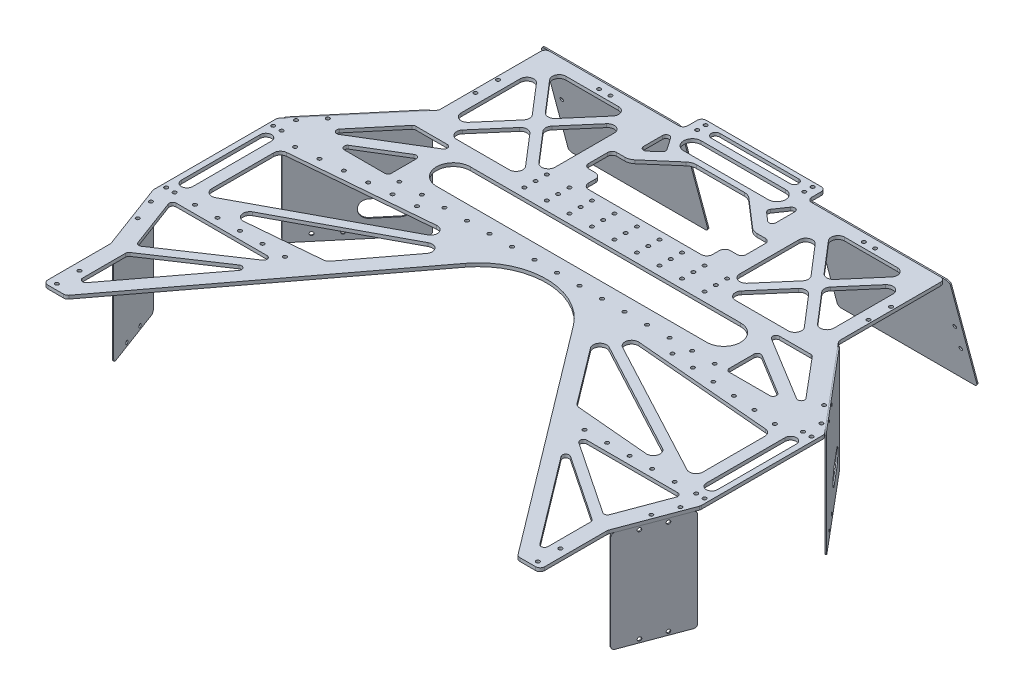
SolidWorks part; units mm, degrees
material "哈碳纤"
ref_plane "前视基准面" through (0, 0, 0) normal (0, 0, 1) x (1, 0, 0)
ref_plane "上视基准面" through (0, 0, 0) normal (0, 1, 0) x (1, 0, 0)
ref_plane "右视基准面" through (0, 0, 0) normal (1, 0, 0) x (0, 0, -1)
other "Configuration Table"
sketch "草图1" plane through (0, 0, 0) normal (0, 1, 0) x (1, 0, 0)
  line L0 (0, -705.937) -> (0, 34590.9145) construction
  line L1 (-55, 0) -> (55, 0)
  line L4 (177.5, -16.4193) -> (177.5, -111)
  line L5 (-177.5, -16.4193) -> (-177.5, -111)
  line L8 (177.5, -111) -> (243, -189)
  line L9 (-177.5, -111) -> (-243, -189)
  line L10 (243, -189) -> (243, -299)
  line L11 (-243, -189) -> (-243, -299)
  line L12 (243, -299) -> (220.55, -359)
  line L13 (-243, -299) -> (-220.55, -359)
  line L14 (220.55, -359) -> (220.55, -419)
  line L15 (-220.55, -359) -> (-220.55, -419)
  line L16 (220.55, -419) -> (200.55, -419)
  line L17 (-220.55, -419) -> (-200.55, -419)
  line L21 (239, -196.5) -> (239, -291.5) construction
  line L22 (-239, -196.5) -> (-239, -291.5) construction
  line L23 (200.55, -419) -> (47.8803, -216.841)
  line L24 (-200.55, -419) -> (-47.8803, -216.841)
  line L25 (234.9875, -309) -> (227.9787, -327.7317) construction
  line L26 (-234.9875, -309) -> (-227.9787, -327.7317) construction
  line L27 (220.3428, -166.684) -> (233.2043, -182) construction
  line L28 (-220.3428, -166.684) -> (-233.2043, -182) construction
  line L29 (217.8171, -159.0112) -> (213.2223, -162.8697) construction
  line L30 (213.2223, -162.8697) -> (234.1223, -187.7582) construction
  line L31 (234.1223, -187.7582) -> (238.7171, -183.8998) construction
  line L33 (55, 0) -> (55, -16.4193)
  line L34 (-55, 0) -> (-55, -16.4193)
  line L35 (55, -16.4193) -> (177.5, -16.4193)
  line L36 (-55, -16.4193) -> (-177.5, -16.4193)
  line L37 (177.5, -16.4193) -> (270.5, -16.4193) construction
  line L38 (270.5, -16.4193) -> (270.5, 8.5) construction
  line L39 (270.5, 8.5) -> (177.5, -16.4193) construction
  line L40 (270.5, -16.4193) -> (273.5, -16.4193) construction
  line L41 (273.5, -16.4193) -> (273.5, -15.6154) construction
  line L42 (273.5, -15.6154) -> (270.5, -16.4193) construction
  circle A0 centre (47.5, -4) radius 1.6
  circle A1 centre (-47.5, -4) radius 1.6
  circle A2 centre (47.5, -11.5) radius 1.6
  circle A3 centre (-47.5, -11.5) radius 1.6
  circle A4 centre (231.5, -196.5) radius 1.6
  circle A5 centre (-231.5, -196.5) radius 1.6
  circle A6 centre (239, -196.5) radius 1.6
  circle A7 centre (-239, -196.5) radius 1.6
  circle A8 centre (231.5, -291.5) radius 1.6
  circle A9 centre (-231.5, -291.5) radius 1.6
  circle A10 centre (239, -291.5) radius 1.6
  circle A11 centre (-239, -291.5) radius 1.6
  arc A12 (47.8803, -216.841) -> (-47.8803, -216.841) centre (0, -253) ccw
  circle A13 centre (213.55, -394) radius 1.6
  circle A14 centre (-213.55, -394) radius 1.6
  circle A15 centre (213.55, -414) radius 1.6
  circle A16 centre (-213.55, -414) radius 1.6
  circle A19 centre (234.9875, -309) radius 1.6
  circle A20 centre (227.9787, -327.7317) radius 1.6
  circle A21 centre (-227.9787, -327.7317) radius 1.6
  circle A22 centre (-234.9875, -309) radius 1.6
  circle A23 centre (220.3428, -166.684) radius 1.6
  circle A24 centre (233.2043, -182) radius 1.6
  circle A25 centre (-233.2043, -182) radius 1.6
  circle A26 centre (-220.3428, -166.684) radius 1.6
  circle A27 centre (112.5, -23.6154) radius 1.6
  circle A28 centre (122.5, -23.6154) radius 1.6
  circle A29 centre (-122.5, -23.6154) radius 1.6
  circle A30 centre (-112.5, -23.6154) radius 1.6
  circle A31 centre (174.5, -61.4193) radius 1.6
  circle A32 centre (174.5, -81.4193) radius 1.6
  circle A33 centre (-174.5, -81.4193) radius 1.6
  circle A34 centre (-174.5, -61.4193) radius 1.6
  point P6 (0, 0)
  point P24 (0, -318.0619)
  point P47 (239, -244)
  point P50 (243, -244)
extrude "凸台-拉伸1" add sketch "草图1" along normal blind 3
sketch "草图2" plane through (311.2944, 0, 116.476) normal (0.9366, 0, 0.3504) x (0.3504, 0, -0.9366)
  line L1 (-196.8824, 0) -> (-256.8824, 0)
  line L2 (-196.8824, 0) -> (-196.8824, -90)
  line L3 (-196.8824, -90) -> (-256.8824, -90)
  line L4 (-256.8824, 0) -> (-256.8824, -90)
  line L5 (-258.9449, 0) -> (-194.8824, 0) construction
  line L7 (-256.8824, -45) -> (-196.8824, -45) construction
  line L8 (-227.0561, 3) -> (-227.0561, 0) construction
  line L9 (-194.8824, 3) -> (-194.8824, 0) construction
  circle A0 centre (-237.0561, -3) radius 1.6
  circle A1 centre (-217.0561, -3) radius 1.6
  circle A2 centre (-217.0561, -87) radius 1.6
  circle A3 centre (-237.0561, -87) radius 1.6
  dimension "D3" = 3
  dimension "D4" = 3.2
  dimension "D1" = 90
  dimension "D2" = 60
  dimension "D5" = 20
  dimension "D6" = 10
  dimension "D7" = 2
extrude "凸台-拉伸2" add sketch "草图2" against normal blind 1 separate body
sketch "草图3" plane through (49.4311, 0, -41.5095) normal (0.7658, 0, -0.6431) x (-0.6431, 0, -0.7658)
  line L0 (-301.0042, 3) -> (-199.1501, 3) construction
  line L1 (-298.0042, 3) -> (-203.0042, 3)
  line L2 (-298.0042, 3) -> (-298.0042, -93)
  line L3 (-298.0042, -93) -> (-203.0042, -93)
  line L4 (-203.0042, 3) -> (-203.0042, -93)
  line L5 (-301.0042, 3) -> (-301.0042, 0) construction
  line L6 (-298.0042, -45) -> (-203.0042, -45) construction
  line L7 (-289.3442, 3) -> (-289.3442, 0) construction
  circle A0 centre (-279.3442, -3) radius 1.6
  circle A1 centre (-259.3442, -3) radius 1.6
  circle A2 centre (-259.3442, -87) radius 1.6
  circle A3 centre (-279.3442, -87) radius 1.6
  dimension "D4" = 6
  dimension "D5" = 3.2
  dimension "D1" = 96
  dimension "D2" = 3
  dimension "D3" = 95
  dimension "D6" = 20
  dimension "D7" = 10
extrude "凸台-拉伸3" add sketch "草图3" along normal blind 1 separate body
sketch "草图6" plane through (177.5, 0, 0) normal (1, 0, 0) x (0, 0, -1)
  line L0 (-16.4193, 3) -> (8.5, -90)
  line L1 (8.5, -90) -> (9.4659, -89.7412)
  line L2 (9.4659, -89.7412) -> (-15.4533, 3.2588)
  line L3 (-15.4533, 3.2588) -> (-16.4193, 3)
  line L4 (-111, 0) -> (-16.4193, 0) construction
  line L6 (-16.4193, 3) -> (-16.4193, 0) construction
  line L7 (-16.4193, 3) -> (-16.4193, 0) construction
  dimension "D1" = 1
  dimension "D2" = 105
  dimension "D3" = 93
extrude "凸台-拉伸5" add sketch "草图6" against normal blind 120 and the other way blind 4 separate body
sketch "草图7" plane through (0, -3.645, 13.6035) normal (0, 0.2588, -0.9659) x (-1, 0, 0)
  line L3 (-122.5, 9.0099) -> (-122.5, 6.1121) construction
  line L4 (-177.5, 4.2496) -> (-55, 4.2496) construction
  line L5 (-181.5, -89.1333) -> (-181.5, 7.1474) construction
  line L7 (-177.5, 7.1474) -> (-55, 7.1474) construction
  circle A0 centre (-122.5, -3.7504) radius 1.6
  circle A1 centre (-112.5, -3.7504) radius 1.6
  circle A2 centre (-174.5, -37.8526) radius 1.6
  circle A3 centre (-174.5, -57.8526) radius 1.6
  dimension "D1" = 10
  dimension "D3" = 3.2
  dimension "D4" = 20
  dimension "D2" = 8
  dimension "D5" = 7
  dimension "D6" = 45
extrude "切除-拉伸2" cut sketch "草图7" against normal blind 1
fillet "圆角1" radius 3 4 edges at (241.8308, 0, 300.698) (220.8045, 0, 356.8931) (241.8308, -90, 300.698) (220.8045, -90, 356.8931)
fillet "圆角2" radius 3 4 edges at (241.4537, 3, 186.3811) (180.3614, 3, 113.6299) (180.3614, -93, 113.6299) (241.4537, -93, 186.3811)
fillet "圆角3" radius 3 4 edges at (181.5, 3.1294, 15.9363) (57.5, -89.8706, -8.983) (57.5, 3.1294, 15.9363) (181.5, -89.8706, -8.983)
sketch "草图9" plane through (50.1969, 0, -42.1526) normal (0.7658, 0, -0.6431) x (-0.6431, 0, -0.7658)
  line L0 (-243.0042, -70) -> (-223.0042, -70) construction
  line L1 (-243.0042, -62.5) -> (-223.0042, -62.5)
  line L2 (-243.0042, -77.5) -> (-223.0042, -77.5)
  line L3 (-203.0042, -90) -> (-203.0042, 0) construction
  line L4 (-295.0042, -93) -> (-206.0042, -93) construction
  arc A0 (-243.0042, -62.5) -> (-243.0042, -77.5) centre (-243.0042, -70) ccw
  arc A1 (-223.0042, -77.5) -> (-223.0042, -62.5) centre (-223.0042, -70) ccw
  point P2 (-233.0042, -70)
  dimension "D1" = 20
  dimension "D2" = 30
  dimension "D3" = 23
  dimension "D4" = 15
extrude "切除-拉伸4" cut sketch "草图9" against normal blind 10
mirror "镜向1" about plane through (0, 0, 0) normal (1, 0, 0) of bodies 107 117 115 109 113
sketch "草图4" plane through (0, 3, 0) normal (0, 1, 0) x (1, 0, 0)
  line L0 (55, 0) -> (-55, 0) construction
  line L1 (-50, -105.5) -> (50, -105.5)
  line L3 (-21.2697, -38.5) -> (21.2697, -38.5)
  line L5 (-55, -105.5) -> (55, -38.5) construction
  line L6 (-55, -38.5) -> (55, -105.5) construction
  line L8 (-70, -85.5) -> (-70, -68.5)
  line L9 (-60, -89.5) -> (-66, -89.5)
  line L11 (-58.7303, -64.5) -> (-66, -64.5)
  line L12 (0, 0) -> (0, -105.5) construction
  line L13 (58.7303, -64.5) -> (66, -64.5)
  line L15 (60, -89.5) -> (66, -89.5)
  line L16 (70, -85.5) -> (70, -68.5)
  line L18 (-52.181, -62.0569) -> (-27.819, -40.9431)
  line L21 (52.181, -62.0569) -> (27.819, -40.9431)
  line L22 (-55, -94.5) -> (-55, -100.5)
  line L23 (55, -94.5) -> (55, -100.5)
  arc A0 (-27.819, -40.9431) -> (-21.2697, -38.5) centre (-21.2697, -48.5) cw
  arc A1 (27.819, -40.9431) -> (21.2697, -38.5) centre (21.2697, -48.5) ccw
  arc A2 (58.7303, -64.5) -> (52.181, -62.0569) centre (58.7303, -54.5) cw
  arc A7 (-52.181, -62.0569) -> (-58.7303, -64.5) centre (-58.7303, -54.5) cw
  arc A8 (66, -64.5) -> (70, -68.5) centre (66, -68.5) cw
  arc A9 (66, -89.5) -> (70, -85.5) centre (66, -85.5) ccw
  arc A10 (-66, -89.5) -> (-70, -85.5) centre (-66, -85.5) cw
  arc A11 (-70, -68.5) -> (-66, -64.5) centre (-66, -68.5) cw
  arc A12 (55, -94.5) -> (60, -89.5) centre (60, -94.5) cw
  arc A13 (55, -100.5) -> (50, -105.5) centre (50, -100.5) cw
  arc A14 (-55, -100.5) -> (-50, -105.5) centre (-50, -100.5) ccw
  arc A15 (-55, -94.5) -> (-60, -89.5) centre (-60, -94.5) ccw
  point P0 (0, -72)
  point P9 (-70, -77)
  point P25 (55, -89.5)
  point P29 (-25, -38.5)
  point P32 (25, -38.5)
  point P35 (55, -64.5)
  point P38 (55, -89.5)
  point P41 (25, -105.5)
  point P44 (-25, -105.5)
  point P46 (-55, -89.5)
  point P47 (-55, -89.5)
  point P50 (-55, -64.5)
  point P53 (70, -64.5)
  point P56 (70, -89.5)
  point P59 (-70, -89.5)
  point P62 (-70, -64.5)
  dimension "D9" = 10
  dimension "D10" = 4
  dimension "D7" = 5
  dimension "D1" = 38.5
  dimension "D2" = 67
  dimension "D3" = 110
  dimension "D4" = 15
  dimension "D5" = 25
  dimension "D6" = 50
  dimension "D8" = 5
extrude "切除-拉伸1" cut sketch "草图4" against normal blind 10
sketch "草图8" plane through (0, 3, 0) normal (0, 1, 0) x (1, 0, 0)
  line L0 (0, 0) -> (0, -193) construction
  line L1 (233, -209) -> (233, -279) construction
  line L2 (238, -209) -> (238, -279)
  line L3 (228, -209) -> (228, -279)
  line L4 (-233, -209) -> (-233, -279) construction
  line L5 (-238, -209) -> (-238, -279)
  line L6 (-228, -209) -> (-228, -279)
  line L7 (243, -299) -> (243, -189) construction
  line L8 (239, -196.5) -> (239, -291.5) construction
  line L9 (-239, -196.5) -> (-239, -291.5) construction
  line L10 (206.55, -398.0824) -> (206.55, -360.0284)
  line L11 (-206.55, -398.0824) -> (-206.55, -360.0284)
  line L12 (209.3187, -346.2133) -> (225.4685, -303.0513)
  line L13 (-209.3187, -346.2133) -> (-225.4685, -303.0513)
  line L14 (222.6588, -299) -> (142.0295, -299)
  line L15 (-222.6588, -299) -> (-142.0295, -299)
  line L16 (143.0376, -322.9324) -> (201.156, -399.8904)
  line L17 (-143.0376, -322.9324) -> (-201.156, -399.8904)
  line L18 (220.55, -359) -> (243, -299) construction
  line L19 (47.8803, -216.841) -> (200.55, -419) construction
  line L20 (220.55, -419) -> (220.55, -359) construction
  line L21 (200.55, -419) -> (220.55, -419) construction
  line L22 (124.964, -299) -> (206.55, -353.613) construction
  line L23 (-124.964, -299) -> (-206.55, -353.613) construction
  line L24 (147.1004, -318.6314) -> (205.2188, -357.5354)
  line L25 (-140.3607, -304.493) -> (-204.8402, -347.655)
  line L26 (140.3607, -304.493) -> (204.8402, -347.655)
  line L27 (-147.1004, -318.6314) -> (-205.2188, -357.5354)
  line L28 (122.7389, -302.324) -> (204.3249, -356.9371) construction
  line L29 (-122.7389, -302.324) -> (-204.3249, -356.9371) construction
  line L30 (-127.189, -295.676) -> (-208.7751, -350.289) construction
  line L31 (127.189, -295.676) -> (208.7751, -350.289) construction
  line L32 (-35, -7.75) -> (35, -7.75) construction
  line L33 (-35, -4) -> (35, -4)
  line L34 (-35, -11.5) -> (35, -11.5)
  line L35 (47.5, -4) -> (47.5, -11.5) construction
  line L36 (-47.5, -4) -> (-47.5, -11.5) construction
  line L37 (55, 0) -> (-55, 0) construction
  line L38 (-37.5, -25.75) -> (37.5, -25.75) construction
  line L39 (-37.5, -18) -> (37.5, -18)
  line L40 (-37.5, -33.5) -> (37.5, -33.5)
  line L41 (21.2697, -38.5) -> (-21.2697, -38.5) construction
  line L42 (53.2627, -29.3274) -> (45.9577, -39.893)
  line L43 (-53.2627, -29.3274) -> (-45.9577, -39.893)
  line L44 (46.4606, -43.8662) -> (53.7655, -50.1972)
  line L45 (-46.4606, -43.8662) -> (-53.7655, -50.1972)
  line L46 (58.7303, -47.9301) -> (58.7303, -31.0335)
  line L47 (-58.7303, -47.9301) -> (-58.7303, -31.0335)
  line L48 (52.181, -62.0569) -> (27.819, -40.9431) construction
  line L49 (178.5, -16.4193) -> (60.5, -16.4193) construction
  line L50 (72.678, -226.4463) -> (109.3516, -275.0081)
  line L52 (113.6167, -277.3694) -> (178.5782, -283.0528)
  line L54 (218, -276.4983) -> (218, -211.5017) construction
  line L56 (212.5134, -211.0305) -> (89.801, -200.4916)
  line L58 (-120, -155.5) -> (120, -155.5) construction
  line L59 (-120, -140.5) -> (120, -140.5)
  line L60 (-120, -170.5) -> (120, -170.5)
  line L61 (177.5, -111) -> (177.5, -16.4193) construction
  line L62 (100.3508, -125.5) -> (147.1492, -125.5)
  line L63 (82, -103.1888) -> (82, -50.7305)
  line L64 (100.3508, -28.4193) -> (147.1492, -28.4193)
  line L65 (165.5, -103.1888) -> (165.5, -50.7305)
  line L66 (82, -125.5) -> (165.5, -28.4193) construction
  line L67 (82, -28.4193) -> (165.5, -125.5) construction
  line L68 (70, -85.5) -> (70, -68.5) construction
  line L69 (95.8019, -115.5875) -> (119.2011, -88.3825)
  line L70 (92.5489, -46.818) -> (115.1088, -73.0471)
  line L71 (92.5489, -107.1013) -> (115.1088, -80.8722)
  line L72 (95.8019, -38.3318) -> (119.2011, -65.5368)
  line L73 (-50, -105.5) -> (50, -105.5) construction
  line L74 (78.9674, -122.8917) -> (162.4674, -25.8109) construction
  line L75 (85.0326, -128.1083) -> (168.5326, -31.0276) construction
  line L76 (78.9674, -31.0276) -> (162.4674, -128.1083) construction
  line L77 (85.0326, -25.8109) -> (168.5326, -122.8917) construction
  line L78 (128.2989, -65.5368) -> (151.6981, -38.3318)
  line L79 (128.2989, -88.3825) -> (151.6981, -115.5875)
  line L80 (132.3912, -80.8722) -> (154.9511, -107.1013)
  line L81 (132.3912, -73.0471) -> (154.9511, -46.818)
  line L82 (-82, -28.4193) -> (-165.5, -125.5) construction
  line L83 (-82, -125.5) -> (-165.5, -28.4193) construction
  line L84 (-132.3912, -73.0471) -> (-154.9511, -46.818)
  line L85 (-132.3912, -80.8722) -> (-154.9511, -107.1013)
  line L86 (-128.2989, -88.3825) -> (-151.6981, -115.5875)
  line L87 (-128.2989, -65.5368) -> (-151.6981, -38.3318)
  line L88 (-95.8019, -38.3318) -> (-119.2011, -65.5368)
  line L89 (-92.5489, -107.1013) -> (-115.1088, -80.8722)
  line L90 (-92.5489, -46.818) -> (-115.1088, -73.0471)
  line L91 (-95.8019, -115.5875) -> (-119.2011, -88.3825)
  line L92 (-165.5, -103.1888) -> (-165.5, -50.7305)
  line L93 (-100.3508, -28.4193) -> (-147.1492, -28.4193)
  line L94 (-82, -103.1888) -> (-82, -50.7305)
  line L95 (-100.3508, -125.5) -> (-147.1492, -125.5)
  line L96 (50.53, -197.1188) -> (209.1749, -281.7915) construction
  line L97 (80.2912, -217.5372) -> (181.9262, -271.7823)
  line L98 (86.4624, -211.7628) -> (209.1749, -277.2575)
  line L99 (52.4134, -193.59) -> (218.8866, -282.4409) construction
  line L100 (48.6465, -200.6477) -> (215.1198, -289.4985) construction
  line L101 (-50.53, -197.1188) -> (-209.1749, -281.7915) construction
  line L102 (-218, -276.4983) -> (-218, -211.5017) construction
  line L103 (218, -217.0085) -> (218, -271.9642)
  line L104 (-218, -217.0085) -> (-218, -271.9642)
  line L105 (-86.4624, -211.7628) -> (-209.1749, -277.2575)
  line L106 (-80.2912, -217.5372) -> (-181.9262, -271.7823)
  line L107 (-212.5134, -211.0305) -> (-89.801, -200.4916)
  line L108 (-113.6167, -277.3694) -> (-178.5782, -283.0528)
  line L109 (-72.678, -226.4463) -> (-109.3516, -275.0081)
  line L110 (50.53, -197.1188) -> (217.0032, -285.9697) construction
  line L111 (-207.0139, -169.4716) -> (-177.7061, -134.5708)
  line L112 (207.0139, -169.4716) -> (177.7061, -134.5708)
  line L113 (-175.4087, -133.5) -> (-147.488, -133.5)
  line L114 (175.4087, -133.5) -> (147.488, -133.5)
  line L115 (-145.926, -139.0613) -> (-203.1545, -173.9621)
  line L116 (145.926, -139.0613) -> (203.1545, -173.9621)
  line L117 (-154.562, -156.0409) -> (-190.4689, -177.9387)
  line L118 (154.562, -156.0409) -> (190.4689, -177.9387)
  line L119 (-188.9069, -183.5) -> (-153, -183.5)
  line L120 (188.9069, -183.5) -> (153, -183.5)
  line L121 (-150, -180.5) -> (-150, -158.6021)
  line L122 (150, -180.5) -> (150, -158.6021)
  line L124 (-181.9077, -116.2489) -> (-239.1415, -184.4052) construction
  arc A0 (47.8803, -216.841) -> (-47.8803, -216.841) centre (0, -253) ccw construction
  arc A1 (238, -209) -> (228, -209) centre (233, -209) ccw
  arc A2 (228, -279) -> (238, -279) centre (233, -279) ccw
  arc A3 (-238, -209) -> (-228, -209) centre (-233, -209) cw
  arc A4 (-228, -279) -> (-238, -279) centre (-233, -279) cw
  arc A5 (205.2188, -357.5354) -> (206.55, -360.0284) centre (203.55, -360.0284) cw
  arc A6 (204.8402, -347.655) -> (209.3187, -346.2133) centre (206.509, -345.162) ccw
  arc A7 (147.1004, -318.6314) -> (143.0376, -322.9324) centre (145.4316, -321.1244) ccw
  arc A8 (-205.2188, -357.5354) -> (-206.55, -360.0284) centre (-203.55, -360.0284) ccw
  arc A9 (-204.8402, -347.655) -> (-209.3187, -346.2133) centre (-206.509, -345.162) cw
  arc A10 (-147.1004, -318.6314) -> (-143.0376, -322.9324) centre (-145.4316, -321.1244) cw
  arc A11 (-142.0295, -299) -> (-140.3607, -304.493) centre (-142.0295, -302) cw
  arc A12 (142.0295, -299) -> (140.3607, -304.493) centre (142.0295, -302) ccw
  arc A13 (225.4685, -303.0513) -> (222.6588, -299) centre (222.6588, -302) ccw
  arc A14 (-225.4685, -303.0513) -> (-222.6588, -299) centre (-222.6588, -302) cw
  arc A15 (-206.55, -398.0824) -> (-201.156, -399.8904) centre (-203.55, -398.0824) ccw
  arc A16 (206.55, -398.0824) -> (201.156, -399.8904) centre (203.55, -398.0824) cw
  arc A17 (-35, -4) -> (-35, -11.5) centre (-35, -7.75) ccw
  arc A18 (35, -11.5) -> (35, -4) centre (35, -7.75) ccw
  arc A19 (-37.5, -18) -> (-37.5, -33.5) centre (-37.5, -25.75) ccw
  arc A20 (37.5, -33.5) -> (37.5, -18) centre (37.5, -25.75) ccw
  arc A21 (-120, -140.5) -> (-120, -170.5) centre (-120, -155.5) ccw
  arc A22 (120, -170.5) -> (120, -140.5) centre (120, -155.5) ccw
  arc A23 (53.7655, -50.1972) -> (58.7303, -47.9301) centre (55.7303, -47.9301) ccw
  arc A24 (53.2627, -29.3274) -> (58.7303, -31.0335) centre (55.7303, -31.0335) cw
  arc A25 (45.9577, -39.893) -> (46.4606, -43.8662) centre (48.4253, -41.5991) ccw
  arc A26 (-45.9577, -39.893) -> (-46.4606, -43.8662) centre (-48.4253, -41.5991) cw
  arc A27 (-53.7655, -50.1972) -> (-58.7303, -47.9301) centre (-55.7303, -47.9301) cw
  arc A28 (-53.2627, -29.3274) -> (-58.7303, -31.0335) centre (-55.7303, -31.0335) ccw
  arc A29 (132.3912, -80.8722) -> (132.3912, -73.0471) centre (136.9401, -76.9596) cw
  arc A30 (128.2989, -88.3825) -> (119.2011, -88.3825) centre (123.75, -92.295) ccw
  arc A31 (115.1088, -80.8722) -> (115.1088, -73.0471) centre (110.5599, -76.9596) ccw
  arc A32 (128.2989, -65.5368) -> (119.2011, -65.5368) centre (123.75, -61.6243) cw
  arc A33 (82, -50.7305) -> (92.5489, -46.818) centre (88, -50.7305) cw
  arc A34 (95.8019, -38.3318) -> (100.3508, -28.4193) centre (100.3508, -34.4193) cw
  arc A35 (147.1492, -28.4193) -> (151.6981, -38.3318) centre (147.1492, -34.4193) cw
  arc A36 (154.9511, -46.818) -> (165.5, -50.7305) centre (159.5, -50.7305) cw
  arc A37 (165.5, -103.1888) -> (154.9511, -107.1013) centre (159.5, -103.1888) cw
  arc A38 (151.6981, -115.5875) -> (147.1492, -125.5) centre (147.1492, -119.5) cw
  arc A39 (95.8019, -115.5875) -> (100.3508, -125.5) centre (100.3508, -119.5) ccw
  arc A40 (92.5489, -107.1013) -> (82, -103.1888) centre (88, -103.1888) cw
  arc A41 (-95.8019, -115.5875) -> (-100.3508, -125.5) centre (-100.3508, -119.5) cw
  arc A42 (-92.5489, -46.818) -> (-82, -50.7305) centre (-88, -50.7305) cw
  arc A43 (-115.1088, -80.8722) -> (-115.1088, -73.0471) centre (-110.5599, -76.9596) cw
  arc A44 (-92.5489, -107.1013) -> (-82, -103.1888) centre (-88, -103.1888) ccw
  arc A45 (-95.8019, -38.3318) -> (-100.3508, -28.4193) centre (-100.3508, -34.4193) ccw
  arc A46 (-151.6981, -38.3318) -> (-147.1492, -28.4193) centre (-147.1492, -34.4193) cw
  arc A47 (-128.2989, -65.5368) -> (-119.2011, -65.5368) centre (-123.75, -61.6243) ccw
  arc A48 (-151.6981, -115.5875) -> (-147.1492, -125.5) centre (-147.1492, -119.5) ccw
  arc A49 (-128.2989, -88.3825) -> (-119.2011, -88.3825) centre (-123.75, -92.295) cw
  arc A50 (-154.9511, -107.1013) -> (-165.5, -103.1888) centre (-159.5, -103.1888) cw
  arc A51 (-154.9511, -46.818) -> (-165.5, -50.7305) centre (-159.5, -50.7305) ccw
  arc A52 (-132.3912, -73.0471) -> (-132.3912, -80.8722) centre (-136.9401, -76.9596) cw
  arc A53 (209.1749, -277.2575) -> (218, -271.9642) centre (212, -271.9642) ccw
  arc A54 (181.9262, -271.7823) -> (178.5782, -283.0528) centre (179.1011, -277.0756) cw
  arc A55 (72.678, -226.4463) -> (80.2912, -217.5372) centre (77.466, -222.8304) cw
  arc A56 (218, -217.0085) -> (212.5134, -211.0305) centre (212, -217.0085) ccw
  arc A57 (86.4624, -211.7628) -> (89.801, -200.4916) centre (89.2876, -206.4695) cw
  arc A58 (218, -276.4983) -> (209.1749, -281.7915) centre (212, -276.4983) cw construction
  arc A59 (109.3516, -275.0081) -> (113.6167, -277.3694) centre (114.1397, -271.3922) ccw
  arc A60 (-113.6167, -277.3694) -> (-109.3516, -275.0081) centre (-114.1397, -271.3922) ccw
  arc A61 (-181.9262, -271.7823) -> (-178.5782, -283.0528) centre (-179.1011, -277.0756) ccw
  arc A62 (-80.2912, -217.5372) -> (-72.678, -226.4463) centre (-77.466, -222.8304) cw
  arc A63 (-86.4624, -211.7628) -> (-89.801, -200.4916) centre (-89.2876, -206.4695) ccw
  arc A64 (-218, -271.9642) -> (-209.1749, -277.2575) centre (-212, -271.9642) ccw
  arc A65 (-212.5134, -211.0305) -> (-218, -217.0085) centre (-212, -217.0085) ccw
  arc A66 (-209.1749, -281.7915) -> (-218, -276.4983) centre (-212, -276.4983) cw construction
  arc A67 (153, -183.5) -> (150, -180.5) centre (153, -180.5) cw
  arc A68 (190.4689, -177.9387) -> (188.9069, -183.5) centre (188.9069, -180.5) cw
  arc A69 (154.562, -156.0409) -> (150, -158.6021) centre (153, -158.6021) ccw
  arc A70 (147.488, -133.5) -> (145.926, -139.0613) centre (147.488, -136.5) ccw
  arc A71 (177.7061, -134.5708) -> (175.4087, -133.5) centre (175.4087, -136.5) ccw
  arc A72 (207.0139, -169.4716) -> (203.1545, -173.9621) centre (204.7165, -171.4009) cw
  arc A73 (-153, -183.5) -> (-150, -180.5) centre (-153, -180.5) ccw
  arc A74 (-190.4689, -177.9387) -> (-188.9069, -183.5) centre (-188.9069, -180.5) ccw
  arc A75 (-154.562, -156.0409) -> (-150, -158.6021) centre (-153, -158.6021) cw
  arc A76 (-147.488, -133.5) -> (-145.926, -139.0613) centre (-147.488, -136.5) cw
  arc A77 (-177.7061, -134.5708) -> (-175.4087, -133.5) centre (-175.4087, -136.5) cw
  arc A78 (-207.0139, -169.4716) -> (-203.1545, -173.9621) centre (-204.7165, -171.4009) ccw
  point P8 (233, -244)
  point P16 (-233, -244)
  point P28 (239, -244)
  point P56 (0, -7.75)
  point P81 (226.9844, -299)
  point P84 (-226.9844, -299)
  point P87 (-206.55, -407.0329)
  point P90 (206.55, -407.0329)
  point P91 (123.75, -76.9596)
  point P103 (47.5, -7.75)
  point P108 (0, -25.75)
  point P128 (218, -244)
  point P136 (0, -155.5)
  point P190 (-123.75, -76.9596)
  point P203 (58.7303, -54.5)
  point P206 (58.7303, -21.4193)
  point P209 (44.4284, -42.105)
  point P212 (-44.4284, -42.105)
  point P215 (-58.7303, -54.5)
  point P218 (-58.7303, -21.4193)
  point P221 (129.026, -76.9596)
  point P224 (123.75, -83.0938)
  point P227 (118.474, -76.9596)
  point P230 (123.75, -70.8255)
  point P233 (82, -34.5534)
  point P236 (87.276, -28.4193)
  point P239 (160.224, -28.4193)
  point P242 (165.5, -34.5534)
  point P245 (165.5, -119.3658)
  point P248 (160.224, -125.5)
  point P251 (87.276, -125.5)
  point P254 (82, -119.3658)
  point P257 (-87.276, -125.5)
  point P260 (-82, -34.5534)
  point P263 (-118.474, -76.9596)
  point P266 (-82, -119.3658)
  point P269 (-87.276, -28.4193)
  point P272 (-160.224, -28.4193)
  point P275 (-123.75, -70.8255)
  point P278 (-160.224, -125.5)
  point P281 (-123.75, -83.0938)
  point P284 (-165.5, -119.3658)
  point P287 (-165.5, -34.5534)
  point P290 (-129.026, -76.9596)
  point P293 (218, -281.9677)
  point P296 (207.8393, -285.6128)
  point P299 (56.2661, -204.7144)
  point P305 (60.6542, -197.9883)
  point P309 (218, -286.5017)
  point P312 (110.9593, -277.1369)
  point P315 (-110.9593, -277.1369)
  point P318 (-207.8393, -285.6128)
  point P321 (-56.2661, -204.7144)
  point P324 (-60.6542, -197.9883)
  point P327 (-218, -281.9677)
  point P333 (-218, -286.5017)
  point P348 (-150, -169.5511)
  point P355 (150, -183.5)
  point P358 (199.5879, -183.5)
  point P361 (150, -153.2587)
  point P364 (136.8069, -133.5)
  point P367 (176.8069, -133.5)
  point P370 (218.7941, -183.5)
  point P373 (-150, -183.5)
  point P376 (-199.5879, -183.5)
  point P379 (-150, -153.2587)
  point P382 (-136.8069, -133.5)
  point P385 (-176.8069, -133.5)
  point P388 (-218.7941, -183.5)
  dimension "D10" = 3
  dimension "D33" = 3
  dimension "D34" = 6
  dimension "D35" = 6
  dimension "D42" = 3
  dimension "D1" = 5
  dimension "D2" = 70
  dimension "D3" = 10
  dimension "D4" = 14
  dimension "D5" = 12
  dimension "D6" = 15
  dimension "D7" = 120
  dimension "D8" = 4
  dimension "D11" = 4
  dimension "D12" = 70
  dimension "D13" = 18
  dimension "D14" = 5
  dimension "D15" = 75
  dimension "D16" = 15
  dimension "D17" = 5
  dimension "D18" = 12
  dimension "D19" = 12
  dimension "D20" = 12
  dimension "D23" = 30
  dimension "D24" = 240
  dimension "D25" = 50
  dimension "D26" = 30
  dimension "D27" = 4
  dimension "D29" = 14
  dimension "D30" = 15
  dimension "D31" = 5
  dimension "D32" = 75
  dimension "D36" = 8
  dimension "D37" = 15
  dimension "D38" = 50
  dimension "D39" = 30
  dimension "D40" = 10
  dimension "D41" = 40
  dimension "D9" = 4
  dimension "D21" = 4
  dimension "D22" = 4
  dimension "D28" = 4
extrude "切除-拉伸3" cut sketch "草图8" against normal blind 10
fillet "圆角4" radius 4 18 edges at (-55, 1.5, 16.4193) (-55, 1.5, 0) (55, 1.5, 0) (55, 1.5, 16.4193) (177.5, 1.5, 16.4193) (177.5, 1.5, 111) (243, 1.5, 189) (243, 1.5, 299) (220.55, 1.5, 359) (200.55, 1.5, 419) (-200.55, 1.5, 419) (-220.55, 1.5, 419) (-220.55, 1.5, 359) (-243, 1.5, 299) (-243, 1.5, 189) (-177.5, 1.5, 111) (-177.5, 1.5, 16.4193) (220.55, 1.5, 419)
sketch "草图10" plane through (0, 3, 0) normal (0, 1, 0) x (1, 0, 0)
  line L0 (0, 0) -> (0, -193) construction
  line L1 (120, -140.5) -> (-120, -140.5) construction
  line L2 (-140, -183.5) -> (-120, -183.5) construction
  line L3 (-120, -170.5) -> (120, -170.5) construction
  line L5 (-213, -292) -> (-193, -292) construction
  line L6 (-142.0295, -299) -> (-222.6588, -299) construction
  line L7 (213, -292) -> (193, -292) construction
  line L8 (-243, -190.4567) -> (-243, -298.2762) construction
  line L9 (-213, -203.0429) -> (-193.0734, -201.3315) construction
  line L10 (-89.801, -200.4916) -> (-212.5134, -211.0305) construction
  line L11 (213, -203.0429) -> (193.0734, -201.3315) construction
  arc A0 (47.8803, -216.841) -> (-47.8803, -216.841) centre (0, -253) ccw construction
  circle A1 centre (-80, -132.5) radius 1.6
  circle A2 centre (-60, -132.5) radius 1.6
  circle A3 centre (-40, -132.5) radius 1.6
  circle A4 centre (-20, -132.5) radius 1.6
  circle A5 centre (0, -132.5) radius 1.6
  circle A6 centre (20, -132.5) radius 1.6
  circle A7 centre (40, -132.5) radius 1.6
  circle A8 centre (60, -132.5) radius 1.6
  circle A9 centre (80, -132.5) radius 1.6
  circle A10 centre (-80, -122.5) radius 1.6
  circle A11 centre (-60, -122.5) radius 1.6
  circle A12 centre (-40, -122.5) radius 1.6
  circle A13 centre (-20, -122.5) radius 1.6
  circle A14 centre (0, -122.5) radius 1.6
  circle A15 centre (20, -122.5) radius 1.6
  circle A16 centre (40, -122.5) radius 1.6
  circle A17 centre (60, -122.5) radius 1.6
  circle A18 centre (80, -122.5) radius 1.6
  circle A19 centre (-80, -112.5) radius 1.6
  circle A20 centre (-60, -112.5) radius 1.6
  circle A21 centre (-40, -112.5) radius 1.6
  circle A22 centre (-20, -112.5) radius 1.6
  circle A23 centre (0, -112.5) radius 1.6
  circle A24 centre (20, -112.5) radius 1.6
  circle A25 centre (40, -112.5) radius 1.6
  circle A26 centre (60, -112.5) radius 1.6
  circle A27 centre (80, -112.5) radius 1.6
  circle A28 centre (-140, -183.5) radius 1.6
  circle A29 centre (-120, -183.5) radius 1.6
  circle A30 centre (-100, -183.5) radius 1.6
  circle A31 centre (-80, -183.5) radius 1.6
  circle A32 centre (-60, -183.5) radius 1.6
  circle A33 centre (-40, -183.5) radius 1.6
  circle A34 centre (-20, -183.5) radius 1.6
  circle A35 centre (0, -183.5) radius 1.6
  circle A36 centre (20, -183.5) radius 1.6
  circle A37 centre (40, -183.5) radius 1.6
  circle A38 centre (60, -183.5) radius 1.6
  circle A39 centre (80, -183.5) radius 1.6
  circle A40 centre (100, -183.5) radius 1.6
  circle A41 centre (120, -183.5) radius 1.6
  circle A42 centre (140, -183.5) radius 1.6
  circle A43 centre (-213, -292) radius 1.6
  circle A44 centre (-193, -292) radius 1.6
  circle A45 centre (-173, -292) radius 1.6
  circle A46 centre (-153, -292) radius 1.6
  circle A47 centre (-133, -292) radius 1.6
  circle A48 centre (133, -292) radius 1.6
  circle A49 centre (153, -292) radius 1.6
  circle A50 centre (173, -292) radius 1.6
  circle A51 centre (193, -292) radius 1.6
  circle A52 centre (213, -292) radius 1.6
  circle A53 centre (-213, -203.0429) radius 1.6
  circle A54 centre (-193.0734, -201.3315) radius 1.6
  circle A55 centre (-173.1467, -199.6201) radius 1.6
  circle A56 centre (-153.2201, -197.9088) radius 1.6
  circle A57 centre (-133.2934, -196.1974) radius 1.6
  circle A58 centre (-113.3668, -194.486) radius 1.6
  circle A59 centre (113.3668, -194.486) radius 1.6
  circle A60 centre (133.2934, -196.1974) radius 1.6
  circle A61 centre (153.2201, -197.9088) radius 1.6
  circle A62 centre (173.1467, -199.6201) radius 1.6
  circle A63 centre (193.0734, -201.3315) radius 1.6
  circle A64 centre (213, -203.0429) radius 1.6
  dimension "D1" = 9
  dimension "D2" = 20
  dimension "D4" = 3.2
  dimension "D7" = 3.2
  dimension "D11" = 3.2
  dimension "D16" = 3.2
  dimension "D3" = 8
  dimension "D6" = 10
  dimension "D9" = 20
  dimension "D10" = 13
  dimension "D12" = 5
  dimension "D13" = 20
  dimension "D14" = 7
  dimension "D15" = 30
  dimension "D18" = 20
  dimension "D19" = 8
  dimension "D20" = 30
  dimension "D5" = 3
  dimension "D8" = 15
  dimension "D17" = 6
extrude "切除-拉伸5" cut sketch "草图10" against normal blind 10
equation "\"D43@草图1\"=\"D42@草图1\"-8.5"
equation "\"D40@草图1\"=8-\"D45@草图1\""
